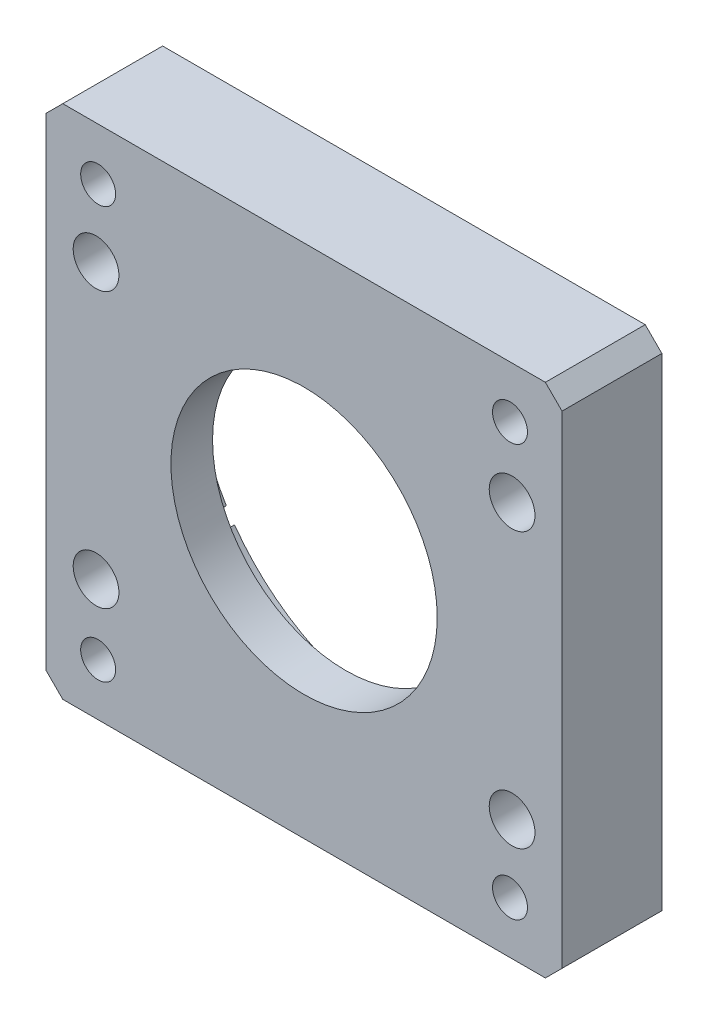
from build123d import *

# Parameters (mm, degrees)
SKETCH_1_W                     = 62
SKETCH_1_H                     = 62
EXTRUDE_1_DEPTH                = 6
SKETCH_2_R                     = 16
CUT_EXTRUDE_1_DEPTH            = 46.453272709
HOLE_WIZARD_M5_1_D             = 4.2
SKETCH_11_R                    = 25
CUT_EXTRUDE_2_DEPTH            = 7
HOLE_WIZARD_M5_1_2_D           = 5.5
HOLE_WIZARD_M5_1_2_CBORE_D     = 10.1
HOLE_WIZARD_M5_1_2_CBORE_DEPTH = 5.4
CHAMFER_1_SIZE                 = 2
SKETCH_13_R                    = 19.2
SKETCH_13_R_2                  = 16.8
CUT_EXTRUDE_3_DEPTH            = 1.5


with BuildPart() as part:
    # 草图1 → 凸台-拉伸1 (new, symmetric)
    with BuildSketch(Plane.XY):
        Rectangle(SKETCH_1_W, SKETCH_1_H)
    extrude(amount=EXTRUDE_1_DEPTH, both=True)

    # 草图2 → 切除-拉伸1 (cut, through all)
    with BuildSketch(Plane.XY.offset(6)):
        Circle(SKETCH_2_R)
    extrude(amount=-CUT_EXTRUDE_1_DEPTH, mode=Mode.SUBTRACT)

    # Hole Wizard M5 _1 (through all)
    with Locations(Plane(origin=(0, 0, -6), x_dir=(1, 0, 0), z_dir=(0, 0, -1))):
        with Locations((-24.748737342, -24.748737342), (24.748737342, -24.748737342), (-24.748737342, 24.748737342), (24.748737342, 24.748737342)):
            Hole(HOLE_WIZARD_M5_1_D / 2)

    # 草图11 → 切除-拉伸2 (cut)
    with BuildSketch(Plane(origin=(0, 0, -6), x_dir=(-1, 0, 0), z_dir=(0, 0, -1))):
        Circle(SKETCH_11_R)
    extrude(amount=-CUT_EXTRUDE_2_DEPTH, mode=Mode.SUBTRACT)

    # Hole Wizard M5 _1 2 (through all)
    with Locations(Plane(origin=(0, 0, -6), x_dir=(-1, 0, 0), z_dir=(0, 0, -1))):
        with Locations((-25, 16.5), (25, 16.5), (25, -16.5), (-25, -16.5)):
            CounterBoreHole(HOLE_WIZARD_M5_1_2_D / 2, HOLE_WIZARD_M5_1_2_CBORE_D / 2, HOLE_WIZARD_M5_1_2_CBORE_DEPTH)

    # 倒角1
    chamfer_1_edges = [part.edges().sort_by_distance(p)[0] for p in [
        (31, -31, 0),
        (-31, -31, 0),
        (-31, 31, 0),
        (31, 31, 0),
    ]]
    chamfer(chamfer_1_edges, length=CHAMFER_1_SIZE)

    # 草图13 → 切除-拉伸3 (cut)
    with BuildSketch(Plane(origin=(0, 0, 1), x_dir=(-1, 0, 0), z_dir=(0, 0, -1))):
        Circle(SKETCH_13_R)
        Circle(SKETCH_13_R_2, mode=Mode.SUBTRACT)
    extrude(amount=-CUT_EXTRUDE_3_DEPTH, mode=Mode.SUBTRACT)


solid = part.part
